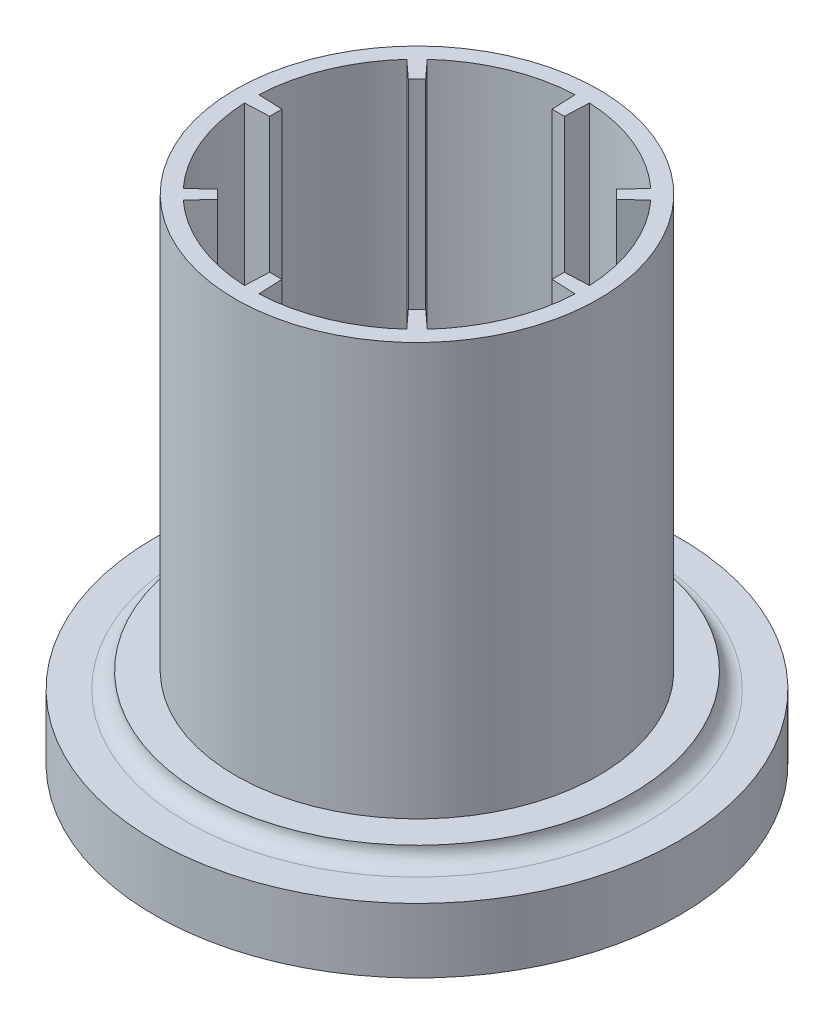
from build123d import *
from build123d.topology import SkipClean

# Parameters (mm, degrees)
REVOLVE_2_ANGLE          = 5.000000000000011
PATTERN_CIRCULAR_1_COUNT = 8
CUT_EXTRUDE_1_REACH      = 583.991
SKETCH_4_R               = 4.999999999999989
SKETCH_4_R_2             = 4.999999999999982
SKETCH_4_R_3             = 4.999999999999985
SKETCH_4_R_4             = 4.999999999999988
SKETCH_4_R_5             = 4.999999999999993
SKETCH_4_R_6             = 4.999999999999983
SKETCH_6_R               = 9.999999999999977
SKETCH_6_R_2             = 9.999999999999979
CUT_EXTRUDE_2_DEPTH      = 260
CUT_EXTRUDE_START        = -180.450361
SKETCH_7_R               = 224.99999999999997
CUT_EXTRUDE_3_DEPTH      = 180.450361
EXTRUDE_START            = 379.63
SKETCH_8_R               = 224.99999999999997
EXTRUDE_1_DEPTH          = 379.63


with BuildPart() as part:
    # 草图1 → 旋转1 (revolve)
    with BuildSketch(Plane.XY):
        with BuildLine():
            Line((-324.99999999999994, 31.77521097831433), (-204.99999999999991, 31.77521097831433))
            Line((-204.99999999999991, 31.77521097831433), (-204.99999999999991, 121.77521097831433))
            ThreePointArc((-204.99999999999991, 121.77521097831433), (-202.0710678118654, 128.84627879017984), (-194.9999999999999, 131.77521097831436))
            Line((-194.9999999999999, 131.77521097831436), (-154.99999999999994, 131.77521097831436))
            ThreePointArc((-154.99999999999994, 131.77521097831436), (-147.92893218813447, 128.8462787901798), (-144.99999999999994, 121.77521097831433))
            Line((-144.99999999999994, 121.77521097831433), (-144.99999999999991, 101.7752109783143))
            Line((-144.99999999999991, 101.7752109783143), (-124.9999999999999, 101.7752109783143))
            Line((-124.9999999999999, 101.7752109783143), (-124.9999999999999, 151.7752109783143))
            Line((-124.9999999999999, 151.7752109783143), (-204.99999999999991, 151.7752109783143))
            Line((-204.99999999999991, 151.7752109783143), (-204.99999999999991, 363.79521097831423))
            Line((-204.99999999999991, 363.79521097831423), (-104.9999999999999, 363.79521097831423))
            Line((-104.9999999999999, 363.79521097831423), (-104.9999999999999, 388.7952109783143))
            Line((-104.9999999999999, 388.7952109783143), (-139.99999999999997, 388.7952109783143))
            Line((-139.99999999999997, 388.7952109783143), (-139.99999999999997, 393.7952109783142))
            Line((-139.99999999999997, 393.7952109783142), (-205, 393.79521097831423))
            Line((-205, 393.79521097831423), (-205, 443.79521097831423))
            Line((-205, 443.79521097831423), (-224.99999999999997, 443.79521097831423))
            Line((-224.99999999999997, 443.79521097831423), (-224.99999999999997, 131.77521097831425))
            Line((-224.99999999999997, 131.77521097831425), (-264.99999999999994, 131.77521097831425))
            ThreePointArc((-264.99999999999994, 131.77521097831425), (-270.85786437626905, 117.63307535458335), (-285, 111.77521097831433))
            Line((-285, 111.77521097831433), (-324.99999999999994, 111.77521097831433))
            Line((-324.99999999999994, 111.77521097831433), (-324.99999999999994, 31.77521097831433))
        make_face()
    revolve(axis=Axis((0, 407.8626331215141, 0), (1.2e-16, -1, 0)))

    # 草图3 → 旋转2 (revolve, symmetric)
    with BuildSketch(Plane.XY) as revolve_2_sk:
        Polygon((-205, 443.79521097831423), (-139.99999999999997, 393.7952109783142), (-205, 393.79521097831423), align=None)
        with BuildLine():
            Line((-104.9999999999999, 363.79521097831423), (-163.0308943816549, 295.8048422932611))
            ThreePointArc((-163.0308943816549, 295.8048422932611), (-171.91239025610793, 280.64304802538896), (-174.9999999999999, 263.3448504181632))
            Line((-174.9999999999999, 263.3448504181632), (-174.99999999999983, 178.9643158667022))
            add(Edge.make_bspline(
                [(-174.99999999999983, 178.9643158667022), (-175.07142129615545, 153.1548036720991), (-154.9999999999999, 136.56500248674672)],
                knots=[0, 0, 0, 1, 1, 1], degree=2))
            Line((-154.9999999999999, 136.56500248674672), (-173.92328032327885, 136.56500248674672))
            Line((-173.92328032327885, 136.56500248674672), (-204.99999999999991, 136.56500248674672))
            Line((-204.99999999999991, 136.56500248674672), (-204.99999999999991, 363.79521097831423))
            Line((-204.99999999999991, 363.79521097831423), (-104.9999999999999, 363.79521097831423))
        make_face()
        with BuildLine():
            Line((-144.99999999999991, 101.7752109783143), (-164.99999999999986, 101.7752109783143))
            Line((-164.99999999999986, 101.7752109783143), (-204.99999999999991, 31.77521097831433))
            Line((-204.99999999999991, 31.77521097831433), (-204.99999999999991, 121.77521097831433))
            ThreePointArc((-204.99999999999991, 121.77521097831433), (-202.0710678118654, 128.84627879017984), (-194.9999999999999, 131.7752109783144))
            Line((-194.9999999999999, 131.7752109783144), (-154.99999999999994, 131.77521097831436))
            ThreePointArc((-154.99999999999994, 131.77521097831436), (-147.92893218813447, 128.8462787901798), (-144.99999999999994, 121.77521097831433))
            Line((-144.99999999999994, 121.77521097831433), (-144.99999999999991, 101.7752109783143))
        make_face()
    revolve_2 = revolve(axis=Axis((0, 407.8626331215141, 0), (1.2e-16, -1, 0)), revolution_arc=REVOLVE_2_ANGLE / 2)
    revolve_2 = revolve_2 + revolve(revolve_2_sk.sketch, axis=Axis((0, 407.8626331215141, 0), (-1.2e-16, 1, 0)), revolution_arc=REVOLVE_2_ANGLE / 2)

    # 阵列(圆周)1: 旋转2 ×8 about axis
    pattern_circular_1_axis = Axis((0, 0, 0), (0, 1, 0))
    for i in range(1, PATTERN_CIRCULAR_1_COUNT):
        add(revolve_2.rotate(pattern_circular_1_axis, i * 360 / PATTERN_CIRCULAR_1_COUNT))

    # 切除-拉伸1: up to this cone (the profile starts outside it)
    cut_extrude_1_end = Plane(origin=(2.34e-15, 388.795211, 0), z_dir=(1.2e-16, -1, 0)).offset(-98.02048294637439) * Cone(1e-06, 653.9417069451008, 766.17357305034, align=(Align.CENTER, Align.CENTER, Align.MIN), mode=Mode.PRIVATE)
    # 草图4 → 切除-拉伸1 (cut, up to the surface)
    with BuildSketch(Plane(origin=(-4.761e-14, 388.7952109783143, 0), x_dir=(1, 1.2e-16, 0), z_dir=(-1.2e-16, 1, 0)), mode=Mode.PRIVATE) as cut_extrude_1_sk1:
        with Locations((115, 0)):
            Circle(SKETCH_4_R)
    cut_extrude_1_tool1 = extrude(cut_extrude_1_sk1.sketch, amount=-CUT_EXTRUDE_1_REACH, mode=Mode.PRIVATE) - cut_extrude_1_end
    add(cut_extrude_1_tool1.solids().sort_by_distance((115, 388.795211, 0))[0], mode=Mode.SUBTRACT)
    # 草图4 → 切除-拉伸1 (cut, up to the surface)
    with BuildSketch(Plane(origin=(-4.761e-14, 388.7952109783143, 0), x_dir=(1, 1.2e-16, 0), z_dir=(-1.2e-16, 1, 0)), mode=Mode.PRIVATE) as cut_extrude_1_sk2:
        with Locations((81.31727983645283, -81.31727983645314)):
            Circle(SKETCH_4_R_2)
    cut_extrude_1_tool2 = extrude(cut_extrude_1_sk2.sketch, amount=-CUT_EXTRUDE_1_REACH, mode=Mode.PRIVATE) - cut_extrude_1_end
    add(cut_extrude_1_tool2.solids().sort_by_distance((81.31728, 388.795211, 81.31728))[0], mode=Mode.SUBTRACT)
    # 草图4 → 切除-拉伸1 (cut, up to the surface)
    with BuildSketch(Plane(origin=(-4.761e-14, 388.7952109783143, 0), x_dir=(1, 1.2e-16, 0), z_dir=(-1.2e-16, 1, 0)), mode=Mode.PRIVATE) as cut_extrude_1_sk3:
        with Locations((-4.0152e-13, -115)):
            Circle(SKETCH_4_R_3)
    cut_extrude_1_tool3 = extrude(cut_extrude_1_sk3.sketch, amount=-CUT_EXTRUDE_1_REACH, mode=Mode.PRIVATE) - cut_extrude_1_end
    add(cut_extrude_1_tool3.solids().sort_by_distance((0, 388.795211, 115))[0], mode=Mode.SUBTRACT)
    # 草图4 → 切除-拉伸1 (cut, up to the surface)
    with BuildSketch(Plane(origin=(-4.761e-14, 388.7952109783143, 0), x_dir=(1, 1.2e-16, 0), z_dir=(-1.2e-16, 1, 0)), mode=Mode.PRIVATE) as cut_extrude_1_sk4:
        with Locations((-81.3172798364534, -81.31727983645251)):
            Circle(SKETCH_4_R_4)
    cut_extrude_1_tool4 = extrude(cut_extrude_1_sk4.sketch, amount=-CUT_EXTRUDE_1_REACH, mode=Mode.PRIVATE) - cut_extrude_1_end
    add(cut_extrude_1_tool4.solids().sort_by_distance((-81.31728, 388.795211, 81.31728))[0], mode=Mode.SUBTRACT)
    # 草图4 → 切除-拉伸1 (cut, up to the surface)
    with BuildSketch(Plane(origin=(-4.761e-14, 388.7952109783143, 0), x_dir=(1, 1.2e-16, 0), z_dir=(-1.2e-16, 1, 0)), mode=Mode.PRIVATE) as cut_extrude_1_sk5:
        with Locations((-115, 8.0304e-13)):
            Circle(SKETCH_4_R_5)
    cut_extrude_1_tool5 = extrude(cut_extrude_1_sk5.sketch, amount=-CUT_EXTRUDE_1_REACH, mode=Mode.PRIVATE) - cut_extrude_1_end
    add(cut_extrude_1_tool5.solids().sort_by_distance((-115, 388.795211, 0))[0], mode=Mode.SUBTRACT)
    # 草图4 → 切除-拉伸1 (cut, up to the surface)
    with BuildSketch(Plane(origin=(-4.761e-14, 388.7952109783143, 0), x_dir=(1, 1.2e-16, 0), z_dir=(-1.2e-16, 1, 0)), mode=Mode.PRIVATE) as cut_extrude_1_sk6:
        with Locations((-81.31727983645226, 81.31727983645371)):
            Circle(SKETCH_4_R_6)
    cut_extrude_1_tool6 = extrude(cut_extrude_1_sk6.sketch, amount=-CUT_EXTRUDE_1_REACH, mode=Mode.PRIVATE) - cut_extrude_1_end
    add(cut_extrude_1_tool6.solids().sort_by_distance((-81.31728, 388.795211, -81.31728))[0], mode=Mode.SUBTRACT)
    # 草图4 → 切除-拉伸1 (cut, up to the surface)
    with BuildSketch(Plane(origin=(-4.761e-14, 388.7952109783143, 0), x_dir=(1, 1.2e-16, 0), z_dir=(-1.2e-16, 1, 0)), mode=Mode.PRIVATE) as cut_extrude_1_sk7:
        with Locations((1.20456e-12, 115)):
            Circle(SKETCH_4_R_4)
    cut_extrude_1_tool7 = extrude(cut_extrude_1_sk7.sketch, amount=-CUT_EXTRUDE_1_REACH, mode=Mode.PRIVATE) - cut_extrude_1_end
    add(cut_extrude_1_tool7.solids().sort_by_distance((0, 388.795211, -115))[0], mode=Mode.SUBTRACT)
    # 草图4 → 切除-拉伸1 (cut, up to the surface)
    with BuildSketch(Plane(origin=(-4.761e-14, 388.7952109783143, 0), x_dir=(1, 1.2e-16, 0), z_dir=(-1.2e-16, 1, 0)), mode=Mode.PRIVATE) as cut_extrude_1_sk8:
        with Locations((81.31727983645395, 81.317279836452)):
            Circle(SKETCH_4_R)
    cut_extrude_1_tool8 = extrude(cut_extrude_1_sk8.sketch, amount=-CUT_EXTRUDE_1_REACH, mode=Mode.PRIVATE) - cut_extrude_1_end
    add(cut_extrude_1_tool8.solids().sort_by_distance((81.31728, 388.795211, -81.31728))[0], mode=Mode.SUBTRACT)

    # 草图6 → 切除-拉伸2 (cut)
    with BuildSketch(Plane(origin=(0, 0, 0), x_dir=(0, -1, 0), z_dir=(-0.3826834323650906, 0, 0.9238795325112865))):
        with Locations((-371.77521097831425, 0)):
            Circle(SKETCH_6_R)
        with Locations(Location((-251.77521097831425, 0, 0), (0, 0, 90))):
            Circle(SKETCH_6_R_2)
    extrude(amount=-CUT_EXTRUDE_2_DEPTH, mode=Mode.SUBTRACT)

    # 草图7 → 切除-拉伸3 (cut)
    with BuildSketch(Plane(origin=(-5.435e-14, 443.79521097831423, 0), x_dir=(1, 1.2e-16, 0), z_dir=(-1.2e-16, 1, 0)).offset(CUT_EXTRUDE_START)):
        with Locations(Location((4.995e-14, 0, 0), (0, 0, 180))):
            Circle(SKETCH_7_R)
    extrude(amount=CUT_EXTRUDE_3_DEPTH, mode=Mode.SUBTRACT)


with BuildPart() as extrude_1_tool:
    # 草图8 → 凸台-拉伸1 (new body)
    with SkipClean():  # the faces are left unmerged after this step: merging them gives an invalid solid
        with BuildSketch(Plane(origin=(-3.225e-14, 263.3448504181632, 0), x_dir=(1, 1.2e-16, 0), z_dir=(-1.2e-16, 1, 0)).offset(EXTRUDE_START)):
            with Locations(Location((4.995e-14, 0, 0), (0, 0, 180))):
                Circle(SKETCH_8_R)
            with BuildLine():
                Line((-204.80488542428068, 8.941974409893897), (-174.83343877682498, 7.633392788933813))
                ThreePointArc((-174.83343877682498, 7.633392788933813), (-174.99999999999986, 2.143e-14), (-174.83343877682498, -7.63339278893381))
                Line((-174.83343877682498, -7.63339278893381), (-204.80488542428068, -8.94197440989384))
                ThreePointArc((-204.80488542428068, -8.94197440989384), (-189.39530416481415, -78.45010363484212), (-151.14185404607704, -138.4959925612084))
                Line((-151.14185404607704, -138.4959925612084), (-129.0235339417731, -118.22828633273882))
                ThreePointArc((-129.0235339417731, -118.22828633273882), (-123.74368670764726, -123.7436867076442), (-118.22828633274202, -129.02353394177015))
                Line((-118.22828633274202, -129.02353394177015), (-138.49599256121215, -151.1418540460736))
                ThreePointArc((-138.49599256121215, -151.1418540460736), (-78.45010363484558, -189.39530416481276), (-8.94197440989605, -204.80488542428063))
                Line((-8.94197440989605, -204.80488542428063), (-7.633392788935682, -174.83343877682483))
                ThreePointArc((-7.633392788935682, -174.83343877682483), (-1.85446e-12, -174.9999999999998), (7.633392788931979, -174.83343877682506))
                Line((7.633392788931979, -174.83343877682506), (8.941974409891698, -204.80488542428088))
                ThreePointArc((8.941974409891698, -204.80488542428088), (78.45010363484155, -189.3953041648145), (138.495992561209, -151.14185404607665))
                Line((138.495992561209, -151.14185404607665), (118.22828633273926, -129.02353394177265))
                ThreePointArc((118.22828633273926, -129.02353394177265), (123.74368670764458, -123.74368670764679), (129.02353394177058, -118.22828633274155))
                Line((129.02353394177058, -118.22828633274155), (151.14185404607417, -138.4959925612117))
                ThreePointArc((151.14185404607417, -138.4959925612117), (189.3953041648134, -78.45010363484425), (204.8048854242808, -8.941974409893902))
                Line((204.8048854242808, -8.941974409893902), (174.83343877682495, -7.633392788933829))
                ThreePointArc((174.83343877682495, -7.633392788933829), (174.99999999999983, -1.093e-14), (174.83343877682498, 7.63339278893381))
                Line((174.83343877682498, 7.63339278893381), (204.80488542428085, 8.9419744098939))
                ThreePointArc((204.80488542428085, 8.9419744098939), (189.39530416481398, 78.45010363484289), (151.14185404607616, 138.4959925612095))
                Line((151.14185404607616, 138.4959925612095), (129.0235339417722, 118.22828633273974))
                ThreePointArc((129.0235339417722, 118.22828633273974), (123.74368670764633, 123.74368670764504), (118.22828633274109, 129.02353394177098))
                Line((118.22828633274109, 129.02353394177098), (138.4959925612111, 151.14185404607468))
                ThreePointArc((138.4959925612111, 151.14185404607468), (78.4501036348442, 189.39530416481338), (8.9419744098946, 204.8048854242807))
                Line((8.9419744098946, 204.8048854242807), (7.633392788934418, 174.8334387768249))
                ThreePointArc((7.633392788934418, 174.8334387768249), (6.3244e-13, 174.9999999999998), (-7.6333927889332, 174.833438776825))
                Line((-7.6333927889332, 174.833438776825), (-8.941974409893167, 204.8048854242808))
                ThreePointArc((-8.941974409893167, 204.8048854242808), (-78.45010363484283, 189.3953041648139), (-138.49599256121, 151.1418540460756))
                Line((-138.49599256121, 151.1418540460756), (-118.22828633274018, 129.02353394177183))
                ThreePointArc((-118.22828633274018, 129.02353394177183), (-123.74368670764548, 123.74368670764594), (-129.02353394177143, 118.22828633274065))
                Line((-129.02353394177143, 118.22828633274065), (-151.1418540460751, 138.4959925612105))
                ThreePointArc((-151.1418540460751, 138.4959925612105), (-189.3953041648136, 78.45010363484347), (-204.80488542428068, 8.941974409893897))
            make_face(mode=Mode.SUBTRACT)
        extrude(amount=-EXTRUDE_1_DEPTH)


with BuildPart() as part_1:
    with SkipClean():  # the faces are left unmerged after this step: merging them gives an invalid solid
        add(part.part)


with BuildPart() as part_2:
    # 凸台-拉伸1: joined with extrude_1_tool
    with SkipClean():  # the faces are left unmerged after this step: merging them gives an invalid solid
        add(part_1.part.fuse(extrude_1_tool.part, tol=0.00001))


solid = part_2.part
